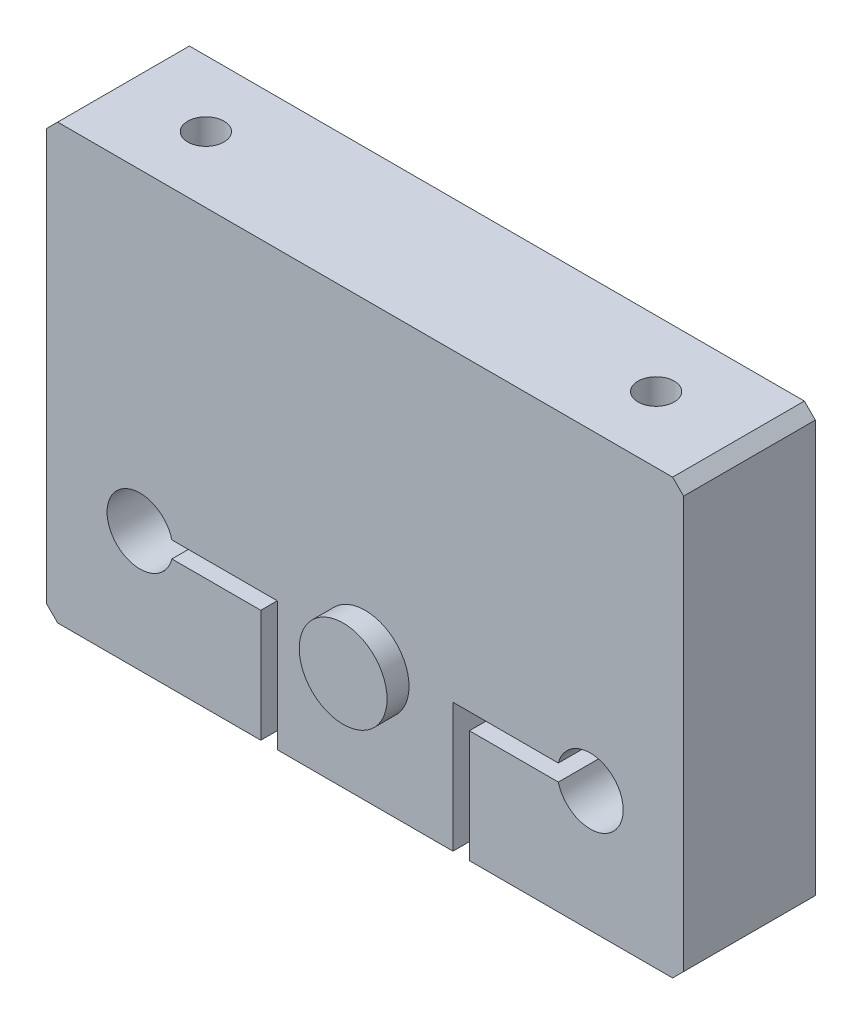
SolidWorks part; units mm, degrees
material "S45C"
ref_plane "Front Plane" through (0, 0, 0) normal (0, 0, 1) x (1, 0, 0)
ref_plane "Top Plane" through (0, 0, 0) normal (0, 1, 0) x (1, 0, 0)
ref_plane "Right Plane" through (0, 0, 0) normal (1, 0, 0) x (0, 0, -1)
sketch "Sketch1" plane through (0, 0, 0) normal (0, 0, 1) x (1, 0, 0)
  line L0 (-17.0609, -8.75) -> (29, -8.75) construction
  line L1 (-29, 19.75) -> (29, 19.75)
  line L2 (-29, 19.75) -> (-29, -19.75)
  line L3 (-29, -19.75) -> (-9.5, -19.75)
  line L4 (29, 19.75) -> (29, -19.75)
  line L5 (-29, 19.75) -> (29, -19.75) construction
  line L6 (-29, -19.75) -> (29, 19.75) construction
  line L7 (-17.5953, -9.5) -> (-9.5, -9.5)
  line L8 (0, 19.75) -> (0, -11) construction
  line L9 (-9.5, -9.5) -> (-9.5, -19.75)
  line L10 (-17.5953, -8) -> (-8, -8)
  line L11 (-8, -8) -> (-8, -19.75)
  line L12 (17.5953, -8) -> (8, -8)
  line L13 (17.5953, -9.5) -> (9.5, -9.5)
  line L14 (8, -8) -> (8, -19.75)
  line L15 (9.5, -9.5) -> (9.5, -19.75)
  line L16 (-8, -19.75) -> (8, -19.75)
  line L17 (9.5, -19.75) -> (29, -19.75)
  arc A0 (-17.5953, -8) -> (-17.5953, -9.5) centre (-20.5, -8.75) ccw
  arc A1 (17.5953, -9.5) -> (17.5953, -8) centre (20.5, -8.75) ccw
  point P0 (0, 0)
  dimension "D3" = 41
  dimension "D5" = 6
  dimension "D8" = 28.5
  dimension "D1" = 39.5
  dimension "D2" = 58
  dimension "D4" = 1.5
  dimension "D6" = 1.5
  dimension "D7" = 16
extrude "Boss-Extrude1" add sketch "Sketch1" along normal mid plane 12
hole_wizard "M4 Tapped Hole1" positions "Sketch3" profile "Sketch2" tap size "M4" standard "GB"
sketch "Sketch3" plane through (0, 19.75, 0) normal (0, 1, 0) x (-1, 0, 0)
  line L0 (0, -6) -> (0, 6) construction
  line L1 (-29, -6) -> (29, -6) construction
  line L2 (-29, 6) -> (29, 6) construction
  point P0 (20.5, 0)
  point P1 (-20.5, 0)
  dimension "D1" = 41
cosmetic thread "Hole thread1" parameters "D1"=8, "D2"=4
cosmetic thread "Hole thread2" parameters "D1"=8, "D2"=4
sketch "Sketch2" plane through (-20.5, 19.75, 0) normal (1, 0, 0) x (0, 0, 1)
  line L0 (0, 0) -> (0, 11.0914)
  line L1 (0, 11.0914) -> (1.65, 10.1)
  line L2 (1.65, 10.1) -> (1.65, 0)
  line L5 (1.65, 0) -> (0, 0)
  line L10 (0, 11.0914) -> (-1.65, 10.1) construction
  line L11 (0, -6.35) -> (0, 107.95) construction
  dimension "螺纹孔钻头直径" = 3.3
  dimension "螺纹孔钻头深度" = 10.1
  dimension "导头角度" = 118
mirror "Mirror1" about plane through (0, 0, 0) normal (0, 1, 0) of "M4 Tapped Hole1"
hole_wizard "CBORE for M3 Hex Head Bolt1" positions "Sketch5" profile "Sketch4" counterbore size "M3" standard "GB"
sketch "Sketch5" plane through (0, -19.75, 0) normal (0, -1, 0) x (1, 0, 0)
  line L0 (0, 6) -> (0, -6) construction
  line L1 (-8, 6) -> (8, 6) construction
  line L2 (-8, -6) -> (8, -6) construction
  point P0 (-13.5, 0)
  point P1 (13.5, 0)
  dimension "D1" = 27
sketch "Sketch4" plane through (-13.5, -19.75, 0) normal (1, 0, 0) x (0, 0, -1)
  line L0 (0, 0) -> (0, 10.25)
  line L1 (0, 10.25) -> (1.75, 10.25)
  line L3 (1.75, 10.25) -> (1.75, 3.5)
  line L4 (1.75, 3.5) -> (3, 3.5)
  line L5 (3, 3.5) -> (3, 0)
  line L7 (3, 0) -> (0, 0)
  line L11 (0, -6.35) -> (0, 107.95) construction
  dimension "通孔孔直径" = 3.5
  dimension "通孔孔深度" = 10.25
  dimension "柱形沉头孔直径" = 6
  dimension "柱形沉头孔深度" = 3.5
hole_wizard "M3 Tapped Hole1" positions "Sketch7" profile "Sketch6" tap size "M3" standard "GB"
sketch "Sketch7" plane through (0, -8, 0) normal (0, -1, 0) x (1, 0, 0)
  point P5 (-13.5, 0)
  point P8 (13.5, 0)
cosmetic thread "Hole thread3" parameters "D1"=6, "D2"=3
cosmetic thread "Hole thread4" parameters "D1"=6, "D2"=3
sketch "Sketch6" plane through (-13.5, -8, 0) normal (1, 0, 0) x (0, 0, -1)
  line L0 (0, 0) -> (0, 8.2511)
  line L1 (0, 8.2511) -> (1.25, 7.5)
  line L2 (1.25, 7.5) -> (1.25, 0)
  line L5 (1.25, 0) -> (0, 0)
  line L10 (0, 8.2511) -> (-1.25, 7.5) construction
  line L11 (0, -6.35) -> (0, 107.95) construction
  dimension "螺纹孔钻头直径" = 2.5
  dimension "螺纹孔钻头深度" = 7.5
  dimension "导头角度" = 118
hole_wizard "M3 Tapped Hole2" positions "Sketch9" profile "Sketch8" tap size "M3" standard "GB"
sketch "Sketch9" plane through (0, -19.75, 0) normal (0, -1, 0) x (1, 0, 0)
  line L0 (9.5, 6) -> (29, 6) construction
  line L1 (29, 6) -> (29, -6) construction
  point P0 (25, 0)
  dimension "D1" = 6
  dimension "D2" = 4
sketch "Sketch8" plane through (25, -19.75, 0) normal (1, 0, 0) x (0, 0, -1)
  line L0 (0, 0) -> (0, 8.7511)
  line L1 (0, 8.7511) -> (1.25, 8)
  line L2 (1.25, 8) -> (1.25, 0)
  line L5 (1.25, 0) -> (0, 0)
  line L10 (0, 8.7511) -> (-1.25, 8) construction
  line L11 (0, -6.35) -> (0, 107.95) construction
  dimension "螺纹孔钻头直径" = 2.5
  dimension "螺纹孔钻头深度" = 8
  dimension "导头角度" = 118
cosmetic thread "Hole thread5" parameters "D1"=6, "D2"=3
sketch "Sketch10" plane through (0, 0, 6) normal (0, 0, 1) x (1, 0, 0)
  line L0 (20.5, -8.75) -> (-20.5, -8.75) construction
  line L2 (-11.4328, -0.535) -> (-11.4328, -0.2762) construction
  circle A0 centre (0, -8.75) radius 4
  dimension "D1" = 8
extrude "Cut-Extrude1" cut sketch "Sketch10" against normal blind 3
sketch "Sketch11" plane through (0, 0, 3) normal (0, 0, 1) x (1, 0, 0)
  circle A0 centre (0, -8.75) radius 4
  circle A1 centre (0, -8.75) radius 4 construction
extrude "Boss-Extrude2" add sketch "Sketch11" along normal blind 5 separate body
chamfer "Chamfer1" distance 1 angle 45 4 edges at (-29, 19.75, 0) (29, 19.75, 0) (29, -19.75, 0) (-29, -19.75, 0)
